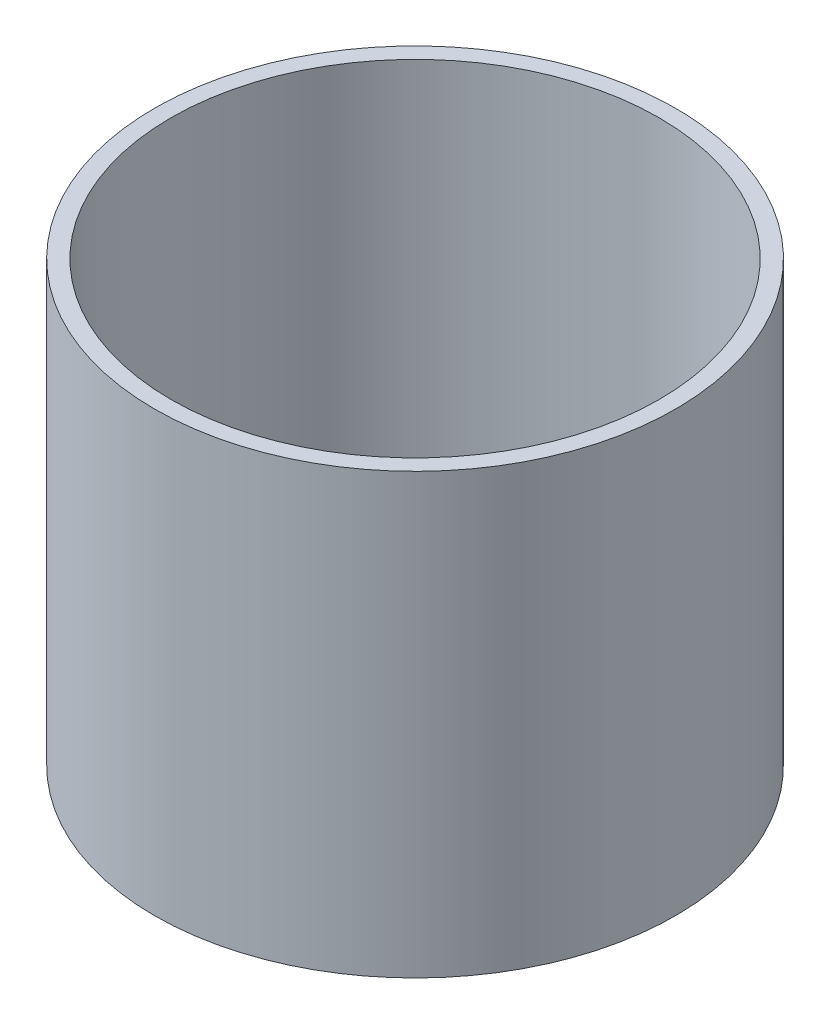
SolidWorks part; units mm, degrees
ref_plane "前视基准面" through (0, 0, 0) normal (0, 0, 1) x (1, 0, 0)
ref_plane "上视基准面" through (0, 0, 0) normal (0, 1, 0) x (1, 0, 0)
ref_plane "右视基准面" through (0, 0, 0) normal (1, 0, 0) x (0, 0, -1)
sketch "草图1" plane through (0, 0, 0) normal (0, 1, 0) x (1, 0, 0)
  circle A0 centre (0, 0) radius 44.5
  circle A1 centre (0, 0) radius 47.5
  dimension "D1" = 95
  dimension "D2" = 89
extrude "凸台-拉伸1" add sketch "草图1" along normal blind 80
